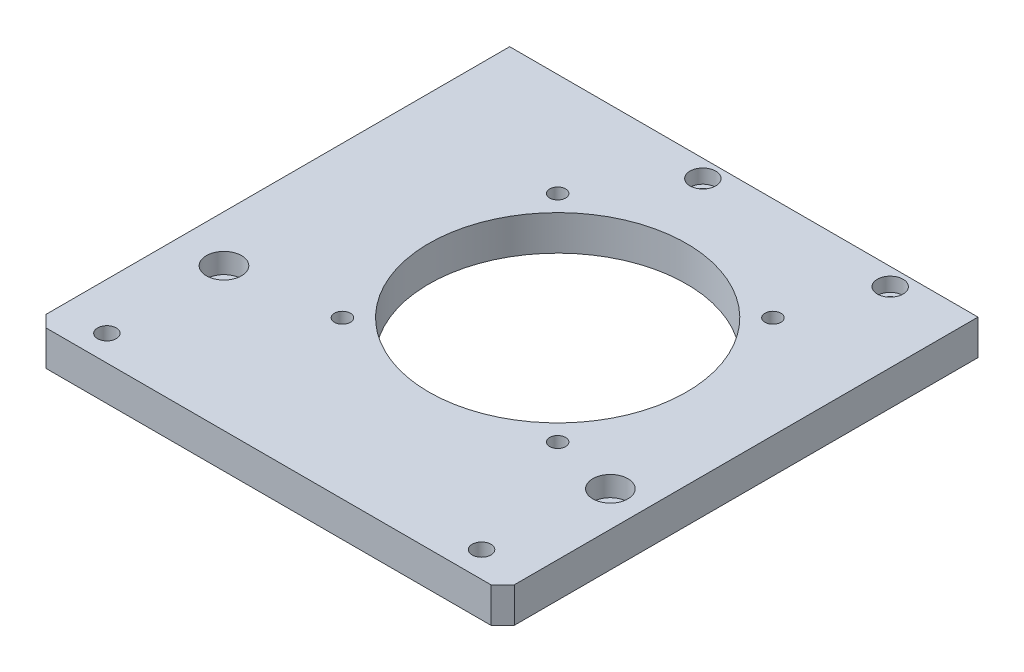
from build123d import *

# Parameters (mm, degrees)
SKETCH1_W                                           = 200
SKETCH1_H                                           = 183
BOSS_EXTRUDE1_DEPTH                                 = 15
M8_TAPPED_HOLE1_D                                   = 6.8
SKETCH11_W                                          = 200
SKETCH11_H                                          = 15
BOSS_EXTRUDE3_DEPTH                                 = 15
CBORE_FOR_M6_HEX_SOCKET_HEAD_CAP_SCREW1_D           = 6.6
CBORE_FOR_M6_HEX_SOCKET_HEAD_CAP_SCREW1_CBORE_D     = 11
CBORE_FOR_M6_HEX_SOCKET_HEAD_CAP_SCREW1_CBORE_DEPTH = 6
CBORE_FOR_M8_HEX_SOCKET_HEAD_CAP_SCREW1_D           = 9
CBORE_FOR_M8_HEX_SOCKET_HEAD_CAP_SCREW1_CBORE_D     = 15
CBORE_FOR_M8_HEX_SOCKET_HEAD_CAP_SCREW1_CBORE_DEPTH = 8.6
SKETCH9_W                                           = 200
SKETCH9_H                                           = 15
BOSS_EXTRUDE2_DEPTH                                 = 5
SKETCH10_R                                          = 4
CUT_EXTRUDE2_DEPTH                                  = 147.857924539
CHAMFER1_SIZE                                       = 5
SKETCH12_R                                          = 55
CUT_EXTRUDE3_DEPTH                                  = 147.857924539


with BuildPart() as part:
    # Sketch1 → Boss-Extrude1 (new body)
    with BuildSketch(Plane(origin=(0, 0, 0), x_dir=(1, 0, 0), z_dir=(0, 1, 0))):
        Rectangle(SKETCH1_W, SKETCH1_H)
    extrude(amount=BOSS_EXTRUDE1_DEPTH)

    # M8 Tapped Hole1 (through all)
    with Locations(Plane(origin=(0, 15, 0), x_dir=(-1, 0, 0), z_dir=(0, 1, 0))):
        with Locations((35.461940777, -62.461940777), (-56.461940777, -62.461940777), (35.461940777, 29.461940777), (-56.461940777, 29.461940777)):
            Hole(M8_TAPPED_HOLE1_D / 2)

    # Sketch11 → Boss-Extrude3 (add)
    with BuildSketch(Plane(origin=(0, 0, -91.5), x_dir=(-1, 0, 0), z_dir=(0, 0, -1))):
        with Locations((0, 7.5)):
            Rectangle(SKETCH11_W, SKETCH11_H)
    extrude(amount=BOSS_EXTRUDE3_DEPTH)

    # CBORE for M6 Hex Socket Head Cap Screw1 (through all)
    with Locations(Plane(origin=(0, 15, 0), x_dir=(-1, 0, 0), z_dir=(0, 1, 0))):
        with Locations((-70, -99), (10, -99)):
            CounterBoreHole(CBORE_FOR_M6_HEX_SOCKET_HEAD_CAP_SCREW1_D / 2, CBORE_FOR_M6_HEX_SOCKET_HEAD_CAP_SCREW1_CBORE_D / 2, CBORE_FOR_M6_HEX_SOCKET_HEAD_CAP_SCREW1_CBORE_DEPTH)

    # CBORE for M8 Hex Socket Head Cap Screw1 (through all)
    with Locations(Plane(origin=(0, 15, 0), x_dir=(-1, 0, 0), z_dir=(0, 1, 0))):
        with Locations((-85, 35.5), (80, 35.5)):
            CounterBoreHole(CBORE_FOR_M8_HEX_SOCKET_HEAD_CAP_SCREW1_D / 2, CBORE_FOR_M8_HEX_SOCKET_HEAD_CAP_SCREW1_CBORE_D / 2, CBORE_FOR_M8_HEX_SOCKET_HEAD_CAP_SCREW1_CBORE_DEPTH)

    # Sketch9 → Boss-Extrude2 (add)
    with BuildSketch(Plane.XY.offset(91.5)):
        with Locations((0, 7.5)):
            Rectangle(SKETCH9_W, SKETCH9_H)
    extrude(amount=BOSS_EXTRUDE2_DEPTH)

    # Sketch10 → Cut-Extrude2 (cut, through all)
    with BuildSketch(Plane(origin=(0, 15, 0), x_dir=(1, 0, 0), z_dir=(0, 1, 0))):
        with Locations(Location((-80, -85.5, 0), (0, 0, 270))):
            Circle(SKETCH10_R)
        with Locations(Location((80, -85.5, 0), (0, 0, 270))):
            Circle(SKETCH10_R)
    extrude(amount=-CUT_EXTRUDE2_DEPTH, mode=Mode.SUBTRACT)

    # Chamfer1
    chamfer1_edges = [part.edges().sort_by_distance(p)[0] for p in [
        (-100, 7.5, 96.5),
        (100, 7.5, 96.5),
    ]]
    chamfer(chamfer1_edges, length=CHAMFER1_SIZE)

    # Sketch12 → Cut-Extrude3 (cut, through all)
    with BuildSketch(Plane(origin=(0, 15, 0), x_dir=(1, 0, 0), z_dir=(0, 1, 0))):
        with Locations(Location((10.5, 16.5, 0), (0, 0, 270))):
            Circle(SKETCH12_R)
    extrude(amount=-CUT_EXTRUDE3_DEPTH, mode=Mode.SUBTRACT)


solid = part.part
